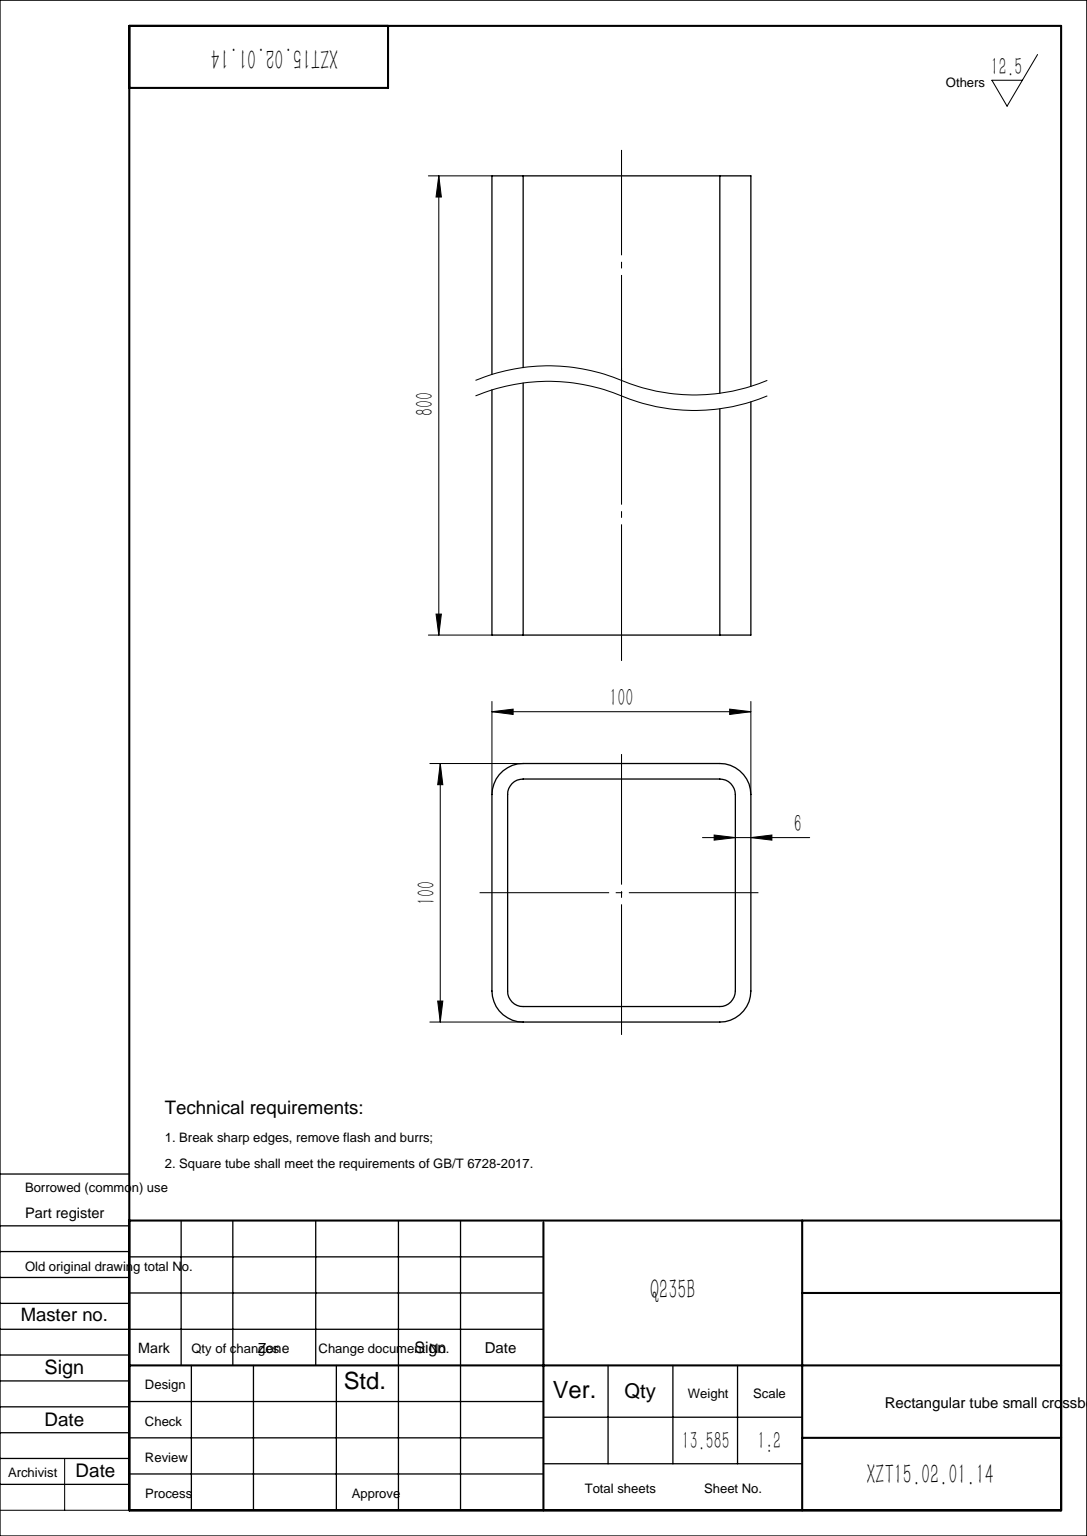
from build123d import *

# Parameters (mm, degrees)
GB_T_6728_2002_SQUARE_HOLLOW_SECTION_100_DEPTH = 800


with BuildPart() as part:
    # Sketch11 → GB/T 6728-2002 square hollow section 100×100×6(1) (new body)
    with BuildSketch(Plane(origin=(0, 0, 0), x_dir=(-1, 0, 0), z_dir=(0, 1, 0))):
        with BuildLine():
            Line((-38, -50), (38, -50))
            ThreePointArc((38, -50), (46.485281374, -46.485281374), (50, -38))
            Line((50, -38), (50, 38))
            ThreePointArc((50, 38), (46.485281374, 46.485281374), (38, 50))
            Line((38, 50), (-38, 50))
            ThreePointArc((-38, 50), (-46.485281374, 46.485281374), (-50, 38))
            Line((-50, 38), (-50, -38))
            ThreePointArc((-50, -38), (-46.485281374, -46.485281374), (-38, -50))
        make_face()
        with BuildLine():
            Line((-38, -44), (38, -44))
            ThreePointArc((38, -44), (42.242640687, -42.242640687), (44, -38))
            Line((44, -38), (44, 38))
            ThreePointArc((44, 38), (42.242640687, 42.242640687), (38, 44))
            Line((38, 44), (-38, 44))
            ThreePointArc((-38, 44), (-42.242640687, 42.242640687), (-44, 38))
            Line((-44, 38), (-44, -38))
            ThreePointArc((-44, -38), (-42.242640687, -42.242640687), (-38, -44))
        make_face(mode=Mode.SUBTRACT)
    extrude(amount=GB_T_6728_2002_SQUARE_HOLLOW_SECTION_100_DEPTH)


solid = part.part
